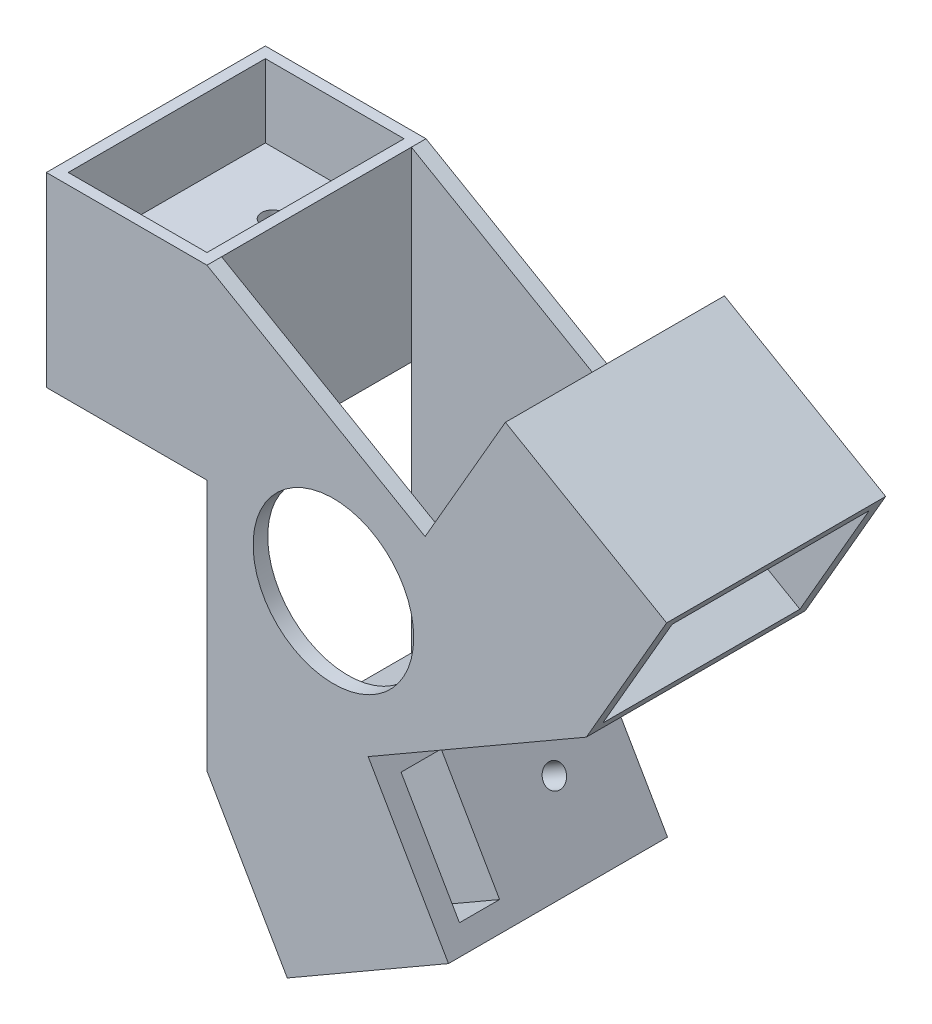
from build123d import *

# Parameters (mm, degrees)
BOSS_EXTRUDE1_DEPTH = 300
CUT_EXTRUDE2_START  = -20
CUT_EXTRUDE2_DEPTH  = 260
SKETCH3_R           = 25
CUT_EXTRUDE3_DEPTH  = 932.86425071
SKETCH4_R           = 15
SKETCH4_W           = 55
SKETCH4_H           = 160
CUT_EXTRUDE4_DEPTH  = 932.86425071
SKETCH5_R           = 15
SKETCH5_W           = 160
SKETCH5_H           = 55
CUT_EXTRUDE5_DEPTH  = 1055.203993494
SKETCH7_R           = 15
SKETCH7_W           = 55
SKETCH7_H           = 160
CUT_EXTRUDE6_DEPTH  = 954.980428731
CUT_EXTRUDE7_REACH  = 933.864
SKETCH8_R           = 110
SKETCH9_W           = 270
SKETCH9_H           = 190
CUT_EXTRUDE8_DEPTH  = 100
CIRPATTERN1_COUNT   = 3


with BuildPart() as part:
    # Sketch1 → Boss-Extrude1 (new body)
    with BuildSketch(Plane.XY):
        Polygon((0, 0), (0, 345), (-220, 345), (-220, 600), (0, 600), (298.778764306, 427.5), (408.778764306, 618.025588833), (629.615242271, 490.525588833), (519.615242271, 300), (220.836477965, 127.5), (330.836477965, -63.025588833), (110, -190.525588833), align=None)
    extrude(amount=BOSS_EXTRUDE1_DEPTH)

    # Sketch2 → Cut-Extrude2 (cut)
    with BuildSketch(Plane(origin=(0, 0, 0), x_dir=(-1, 0, 0), z_dir=(0, 0, -1)).offset(CUT_EXTRUDE2_START)):
        Polygon((0, 600), (0, 0), (-519.615242271, 300), align=None)
    extrude(amount=-CUT_EXTRUDE2_DEPTH, mode=Mode.SUBTRACT)

    # Sketch3 → Cut-Extrude3 (cut, through all)
    with BuildSketch(Plane(origin=(0, 0, 0), x_dir=(-1, 0, 0), z_dir=(0, 0, -1))):
        with Locations((-173.205080757, 300)):
            Circle(SKETCH3_R)
    extrude(amount=-CUT_EXTRUDE3_DEPTH, mode=Mode.SUBTRACT)

    # Sketch4 → Cut-Extrude4 (cut, through all)
    with BuildSketch(Plane(origin=(0, 0, 0), x_dir=(0, 0, 1), z_dir=(-0.866025403784456, -0.4999999999999701, 0))):
        with Locations(Location((100, -110, 0), (0, 0, 270))):
            Circle(SKETCH4_R)
        with Locations((242.5, -110)):
            Rectangle(SKETCH4_W, SKETCH4_H)
    extrude(amount=-CUT_EXTRUDE4_DEPTH, mode=Mode.SUBTRACT)

    # Sketch5 → Cut-Extrude5 (cut, through all)
    with BuildSketch(Plane(origin=(0, 600, 0), x_dir=(1, 0, 0), z_dir=(0, 1, 0))):
        with Locations(Location((-110, -100, 0), (0, 0, 180))):
            Circle(SKETCH5_R)
        with Locations((-110, -242.5)):
            Rectangle(SKETCH5_W, SKETCH5_H)
    extrude(amount=-CUT_EXTRUDE5_DEPTH, mode=Mode.SUBTRACT)

    # Sketch7 → Cut-Extrude6 (cut, through all)
    with BuildSketch(Plane(origin=(259.807621135, -150, 0), x_dir=(0, 0, -1), z_dir=(0.8660254037844342, -0.5000000000000079, 0))):
        with Locations(Location((-100, 629.615242271, 0), (0, 0, 90))):
            Circle(SKETCH7_R)
        with Locations((-242.5, 629.615242271)):
            Rectangle(SKETCH7_W, SKETCH7_H)
    extrude(amount=-CUT_EXTRUDE6_DEPTH, mode=Mode.SUBTRACT)

    # Sketch8 → Cut-Extrude7 (cut, up to next)
    with BuildSketch(Plane.XY.offset(300), mode=Mode.PRIVATE) as cut_extrude7_sk1:
        with Locations((173.205080757, 300)):
            Circle(SKETCH8_R)
    cut_extrude7_tool1 = extrude(cut_extrude7_sk1.sketch, amount=-CUT_EXTRUDE7_REACH, mode=Mode.PRIVATE) & part.part
    add(cut_extrude7_tool1.solids().sort_by_distance((173.205081, 300, 300))[0], mode=Mode.SUBTRACT)

    # Sketch9 → Cut-Extrude8 (cut)
    with BuildSketch(Plane(origin=(0, 0, 0), x_dir=(0, 0, 1), z_dir=(-0.866025403784456, -0.4999999999999701, 0))):
        with Locations((150, -110)):
            Rectangle(SKETCH9_W, SKETCH9_H)
    cut_extrude8 = extrude(amount=-CUT_EXTRUDE8_DEPTH, mode=Mode.SUBTRACT)

    # CirPattern1: Cut-Extrude8 ×3 about axis
    cirpattern1_axis = Axis((173.205080757, 300, 0), (0, 0, 1))
    for i in range(1, CIRPATTERN1_COUNT):
        add(cut_extrude8.rotate(cirpattern1_axis, i * 360 / CIRPATTERN1_COUNT), mode=Mode.SUBTRACT)


solid = part.part
